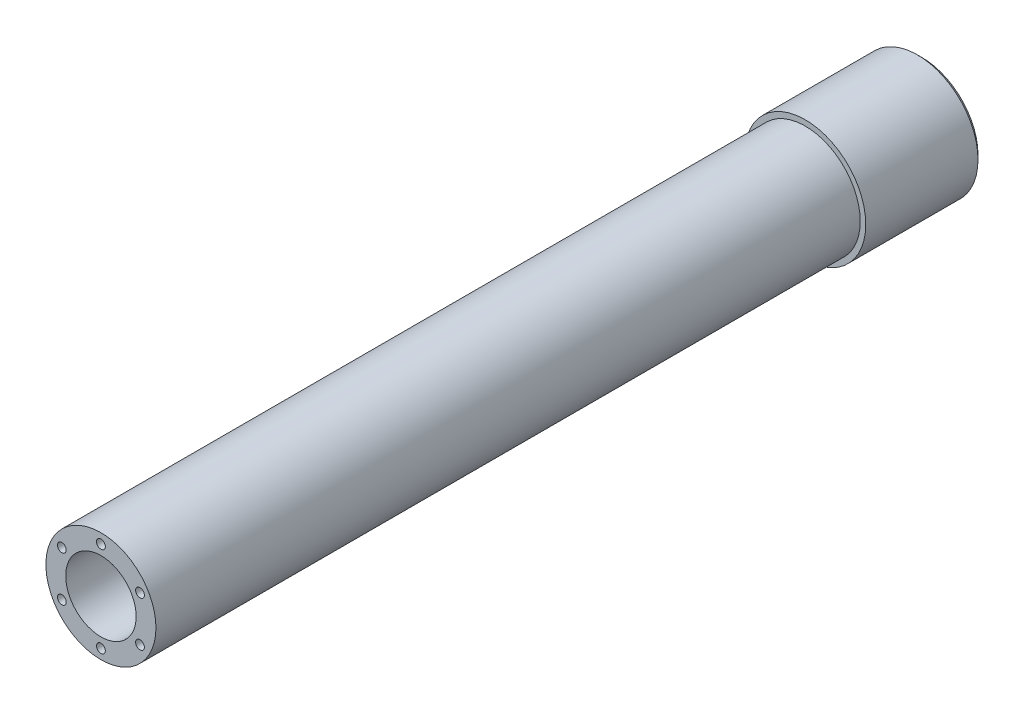
from build123d import *

# Parameters (mm, degrees)
SKETCH1_R           = 27.5
SKETCH1_R_2         = 16
BOSS_EXTRUDE1_DEPTH = 53
SKETCH2_R           = 25
SKETCH2_R_2         = 16
BOSS_EXTRUDE2_DEPTH = 70
SKETCH3_R           = 2
CUT_EXTRUDE1_DEPTH  = 15
CHAMFER1_SIZE       = 2
SKETCH4_R           = 25
SKETCH4_R_2         = 16
BOSS_EXTRUDE3_DEPTH = 250
SKETCH5_R           = 2
CUT_EXTRUDE2_DEPTH  = 12


with BuildPart() as part:
    # Sketch1 → Boss-Extrude1 (new body)
    with BuildSketch(Plane.XY):
        Circle(SKETCH1_R)
        Circle(SKETCH1_R_2, mode=Mode.SUBTRACT)
    extrude(amount=BOSS_EXTRUDE1_DEPTH)

    # Sketch2 → Boss-Extrude2 (add)
    with BuildSketch(Plane.XY.offset(53)):
        Circle(SKETCH2_R)
        Circle(SKETCH2_R_2, mode=Mode.SUBTRACT)
    extrude(amount=BOSS_EXTRUDE2_DEPTH)

    # Sketch3 → Cut-Extrude1 (cut)
    with BuildSketch(Plane(origin=(0, 0, 0), x_dir=(-1, 0, 0), z_dir=(0, 0, -1))):
        with Locations((0, 19)):
            Circle(SKETCH3_R)
        with Locations((13.435028843, 13.435028843)):
            Circle(SKETCH3_R)
        with Locations((19, 0)):
            Circle(SKETCH3_R)
        with Locations((13.435028843, -13.435028843)):
            Circle(SKETCH3_R)
        with Locations((0, -19)):
            Circle(SKETCH3_R)
        with Locations((-13.435028843, -13.435028843)):
            Circle(SKETCH3_R)
        with Locations((-19, 0)):
            Circle(SKETCH3_R)
        with Locations((-13.435028843, 13.435028843)):
            Circle(SKETCH3_R)
    extrude(amount=-CUT_EXTRUDE1_DEPTH, mode=Mode.SUBTRACT)

    # Chamfer1
    chamfer1_edges = [part.edges().sort_by_distance(p)[0] for p in [
        (-27.5, 0, 0),
    ]]
    chamfer(chamfer1_edges, length=CHAMFER1_SIZE)

    # Sketch4 → Boss-Extrude3 (add)
    with BuildSketch(Plane.XY.offset(123)):
        Circle(SKETCH4_R)
        Circle(SKETCH4_R_2, mode=Mode.SUBTRACT)
    extrude(amount=BOSS_EXTRUDE3_DEPTH)

    # Sketch5 → Cut-Extrude2 (cut)
    with BuildSketch(Plane.XY.offset(373)):
        with Locations((0, 20.5)):
            Circle(SKETCH5_R)
        with Locations((17.753520778, 10.25)):
            Circle(SKETCH5_R)
        with Locations((17.753520778, -10.25)):
            Circle(SKETCH5_R)
        with Locations((0, -20.5)):
            Circle(SKETCH5_R)
        with Locations((-17.753520778, -10.25)):
            Circle(SKETCH5_R)
        with Locations((-17.753520778, 10.25)):
            Circle(SKETCH5_R)
    extrude(amount=-CUT_EXTRUDE2_DEPTH, mode=Mode.SUBTRACT)


solid = part.part
